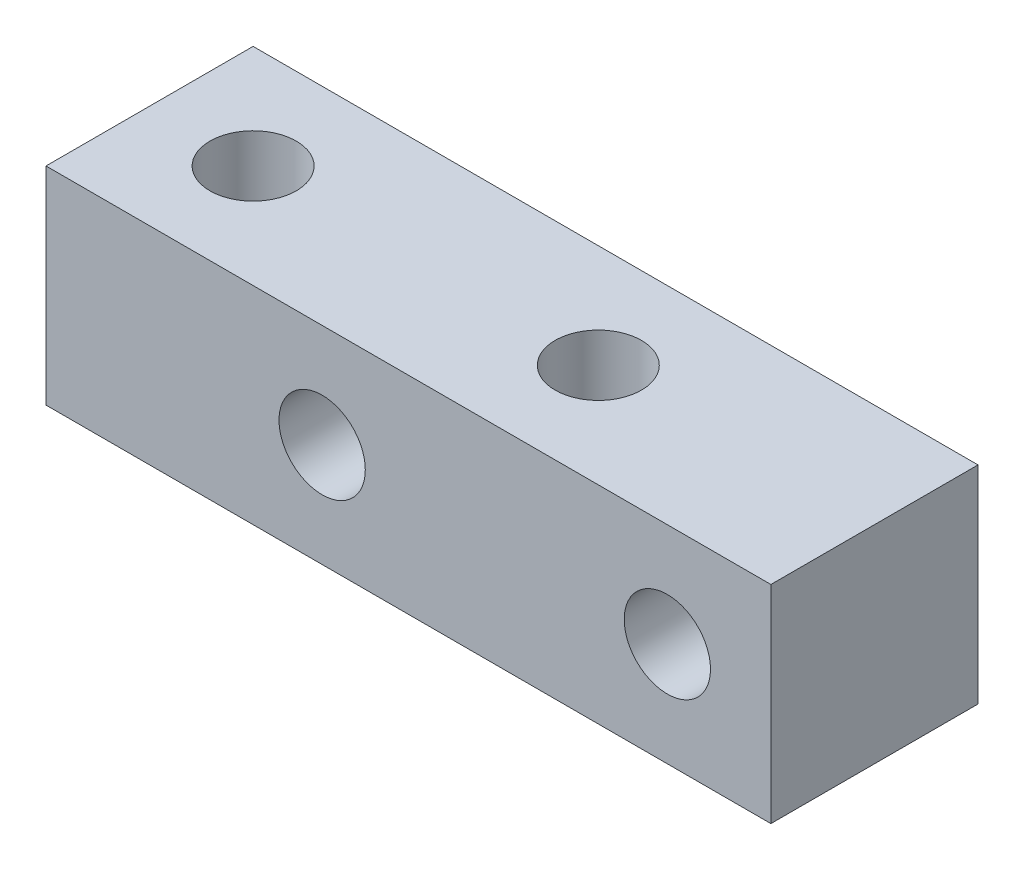
from build123d import *

# Parameters (mm, degrees)
SKETCH_1_W         = 21
SKETCH_1_H         = 6
EXTRUDE_1_DEPTH    = 6
HOLE_WIZARD_M3_1_D = 2.5
HOLE_WIZARD_M3_2_D = 2.5


with BuildPart() as part:
    # 草图1 → 凸台-拉伸1 (new body)
    with BuildSketch(Plane(origin=(0, 0, 0), x_dir=(1, 0, 0), z_dir=(0, 1, 0))):
        Rectangle(SKETCH_1_W, SKETCH_1_H)
    extrude(amount=EXTRUDE_1_DEPTH)

    # M3 螺纹孔1 (through all)
    with Locations(Plane.XY.offset(3)):
        with Locations((-2.5, 3), (7.5, 3)):
            Hole(HOLE_WIZARD_M3_1_D / 2)

    # M3 螺纹孔2 (through all)
    with Locations(Plane(origin=(0, 6, 0), x_dir=(1, 0, 0), z_dir=(0, 1, 0))):
        with Locations((2.5, 0), (-7.5, 0)):
            Hole(HOLE_WIZARD_M3_2_D / 2)


solid = part.part
